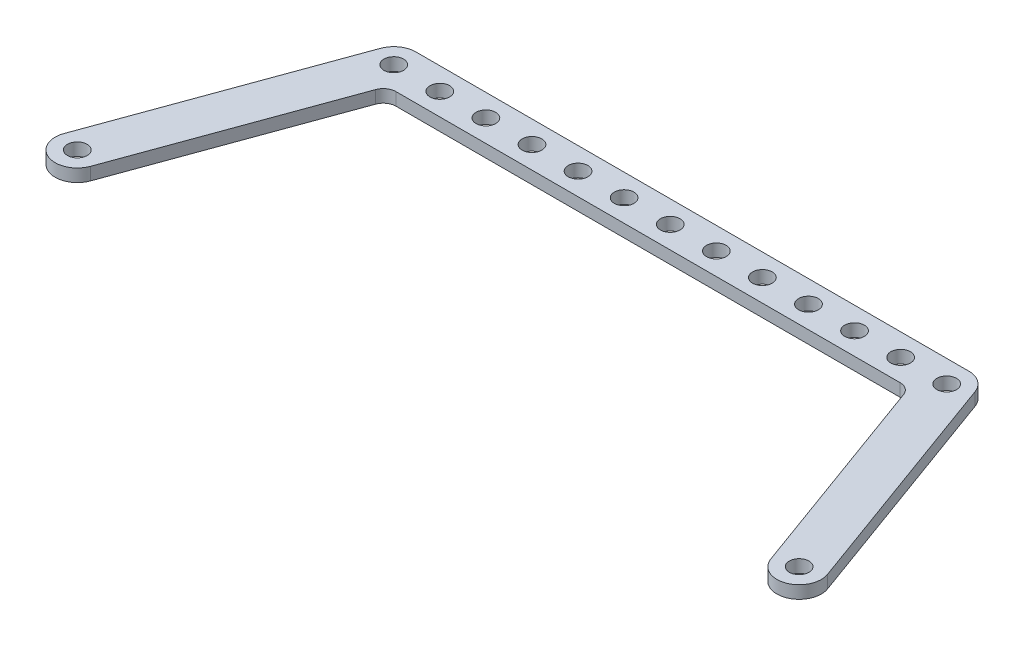
from build123d import *

# Parameters (mm, degrees)
SKETCH_1_R      = 1.55
EXTRUDE_1_DEPTH = 2
FILLET_1_R      = 2


with BuildPart() as part:
    # 草图1 → 凸台-拉伸1 (new body)
    with BuildSketch(Plane(origin=(0, 0, 0), x_dir=(1, 0, 0), z_dir=(0, 1, 0))):
        with BuildLine():
            Line((41.213806874, 33.138893752), (53.711075827, -1.197070502))
            ThreePointArc((53.711075827, -1.197070502), (58.197070502, -3.288924173), (60.288924173, 1.197070502))
            Line((60.288924173, 1.197070502), (46.953457431, 37.835964254))
            ThreePointArc((46.953457431, 37.835964254), (45.672050785, 39.505925907), (43.664533258, 40.138893752))
            Line((43.664533258, 40.138893752), (-43.664533258, 40.138893752))
            ThreePointArc((-43.664533258, 40.138893752), (-45.672050785, 39.505925907), (-46.953457431, 37.835964254))
            Line((-46.953457431, 37.835964254), (-60.288924173, 1.197070502))
            ThreePointArc((-60.288924173, 1.197070502), (-58.197070502, -3.288924173), (-53.711075827, -1.197070502))
            Line((-53.711075827, -1.197070502), (-41.213806874, 33.138893752))
            Line((-41.213806874, 33.138893752), (41.213806874, 33.138893752))
        make_face()
        with Locations(Location((43.664533258, 36.638893752, 0), (0, 0, 270))):
            Circle(SKETCH_1_R, mode=Mode.SUBTRACT)
        with Locations(Location((57, 0, 0), (0, 0, 270))):
            Circle(SKETCH_1_R, mode=Mode.SUBTRACT)
        with Locations(Location((29.110533258, 36.638893752, 0), (0, 0, 270))):
            Circle(SKETCH_1_R, mode=Mode.SUBTRACT)
        with Locations(Location((36.387533258, 36.638893752, 0), (0, 0, 270))):
            Circle(SKETCH_1_R, mode=Mode.SUBTRACT)
        with Locations(Location((-36.387533258, 36.638893752, 0), (0, 0, 270))):
            Circle(SKETCH_1_R, mode=Mode.SUBTRACT)
        with Locations(Location((-29.110533258, 36.638893752, 0), (0, 0, 270))):
            Circle(SKETCH_1_R, mode=Mode.SUBTRACT)
        with Locations(Location((-21.833533258, 36.638893752, 0), (0, 0, 270))):
            Circle(SKETCH_1_R, mode=Mode.SUBTRACT)
        with Locations(Location((-14.556533258, 36.638893752, 0), (0, 0, 270))):
            Circle(SKETCH_1_R, mode=Mode.SUBTRACT)
        with Locations(Location((-7.279533258, 36.638893752, 0), (0, 0, 270))):
            Circle(SKETCH_1_R, mode=Mode.SUBTRACT)
        with Locations(Location((0, 36.638893752, 0), (0, 0, 270))):
            Circle(SKETCH_1_R, mode=Mode.SUBTRACT)
        with Locations(Location((7.279533258, 36.638893752, 0), (0, 0, 270))):
            Circle(SKETCH_1_R, mode=Mode.SUBTRACT)
        with Locations(Location((14.556533258, 36.638893752, 0), (0, 0, 270))):
            Circle(SKETCH_1_R, mode=Mode.SUBTRACT)
        with Locations(Location((21.833533258, 36.638893752, 0), (0, 0, 270))):
            Circle(SKETCH_1_R, mode=Mode.SUBTRACT)
        with Locations(Location((-43.664533258, 36.638893752, 0), (0, 0, 270))):
            Circle(SKETCH_1_R, mode=Mode.SUBTRACT)
        with Locations(Location((-57, 0, 0), (0, 0, 270))):
            Circle(SKETCH_1_R, mode=Mode.SUBTRACT)
    extrude(amount=EXTRUDE_1_DEPTH)

    # 圆角1
    fillet_1_edges = [part.edges().sort_by_distance(p)[0] for p in [
        (-41.213806874, 1, -33.138893752),
        (41.213806874, 1, -33.138893752),
    ]]
    fillet(fillet_1_edges, radius=FILLET_1_R)


solid = part.part
